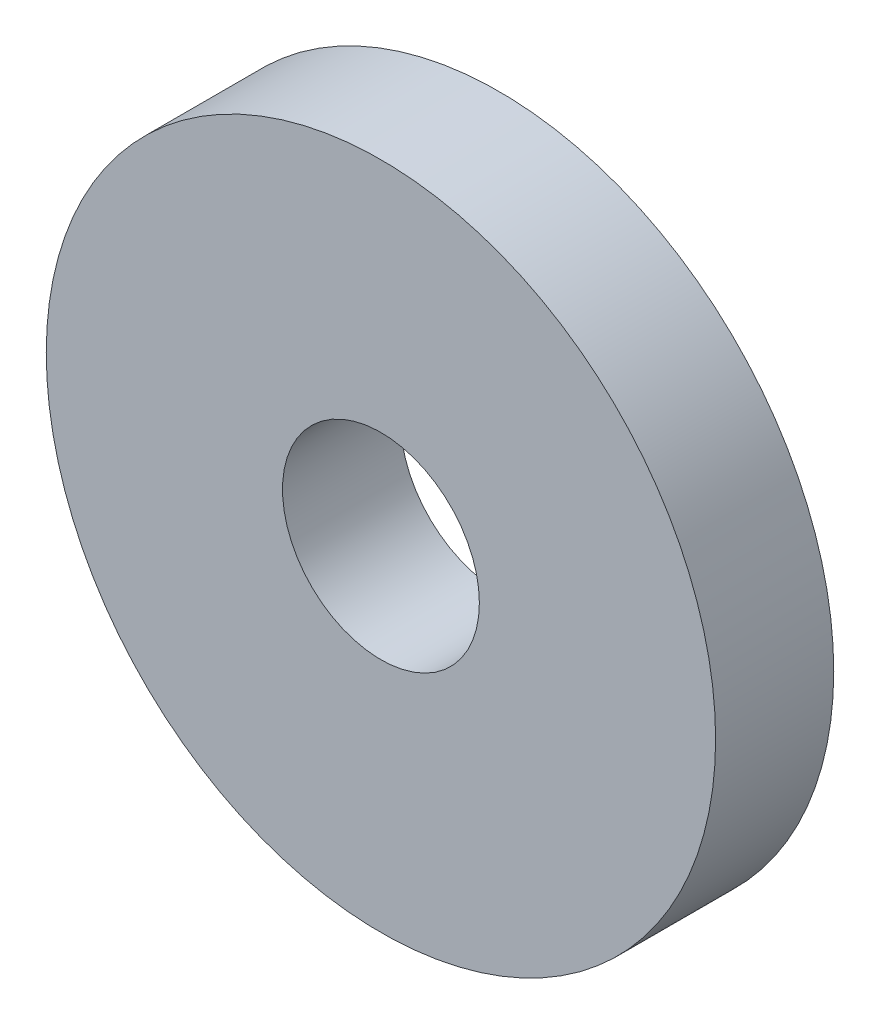
SolidWorks part; units mm, degrees
ref_plane "Front Plane" through (0, 0, 0) normal (0, 0, 1) x (1, 0, 0)
ref_plane "Top Plane" through (0, 0, 0) normal (0, 1, 0) x (1, 0, 0)
ref_plane "Right Plane" through (0, 0, 0) normal (1, 0, 0) x (0, 0, -1)
other "Configuration Table"
sketch "Sketch1" plane through (0, 0, 0) normal (0, 0, 1) x (1, 0, 0)
  circle A0 centre (0, 0) radius 85
  circle A2 centre (0, 0) radius 25
extrude "Boss-Extrude1" add sketch "Sketch1" along normal blind 30
